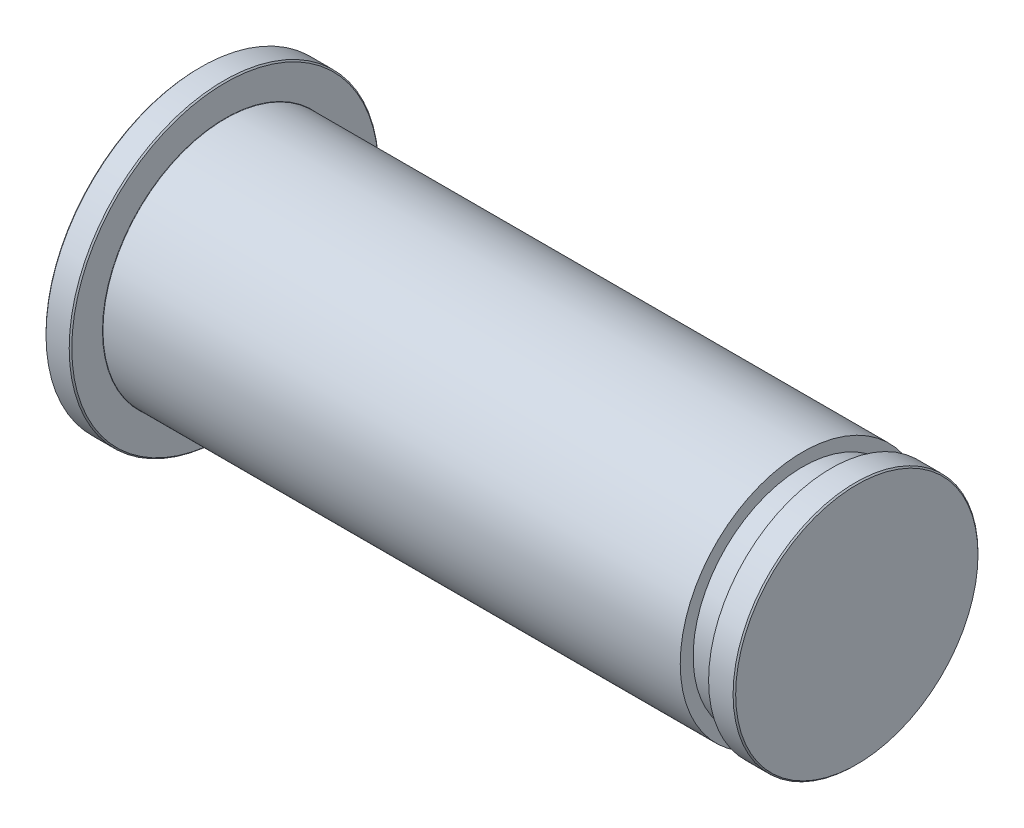
from build123d import *

# Parameters (mm, degrees)
SKETCH1_R           = 4.75
BOSS_EXTRUDE1_DEPTH = 24.5
SKETCH2_R           = 6
BOSS_EXTRUDE2_DEPTH = 1
CHAMFER1_SIZE       = 0.05
FILLET1_R           = 0.01
CHAMFER2_SIZE       = 0.05
SKETCH4_R           = 5.5
SKETCH4_R_2         = 4.25
CUT_EXTRUDE1_DEPTH  = 1.1


with BuildPart() as part:
    # Sketch1 → Boss-Extrude1 (new body)
    with BuildSketch(Plane(origin=(0, 0, 0), x_dir=(0, 0, -1), z_dir=(1, 0, 0))):
        Circle(SKETCH1_R)
    extrude(amount=BOSS_EXTRUDE1_DEPTH)

    # Sketch2 → Boss-Extrude2 (add)
    with BuildSketch(Plane.ZY):
        Circle(SKETCH2_R)
    extrude(amount=BOSS_EXTRUDE2_DEPTH)

    # Chamfer1
    chamfer1_edges = [part.edges().sort_by_distance(p)[0] for p in [
        (0, 0, -6),
        (-1, 0, -6),
    ]]
    chamfer(chamfer1_edges, length=CHAMFER1_SIZE)

    # Fillet1
    fillet1_edges = [part.edges().sort_by_distance(p)[0] for p in [
        (0, 0, 4.75),
    ]]
    fillet(fillet1_edges, radius=FILLET1_R)

    # Chamfer2
    chamfer2_edges = [part.edges().sort_by_distance(p)[0] for p in [
        (24.5, 0, 4.75),
    ]]
    chamfer(chamfer2_edges, length=CHAMFER2_SIZE)

    # Sketch4 → Cut-Extrude1 (cut)
    with BuildSketch(Plane(origin=(23.5, 0, 0), x_dir=(0, 0, -1), z_dir=(1, 0, 0))):
        Circle(SKETCH4_R)
        Circle(SKETCH4_R_2, mode=Mode.SUBTRACT)
    extrude(amount=-CUT_EXTRUDE1_DEPTH, mode=Mode.SUBTRACT)


solid = part.part
